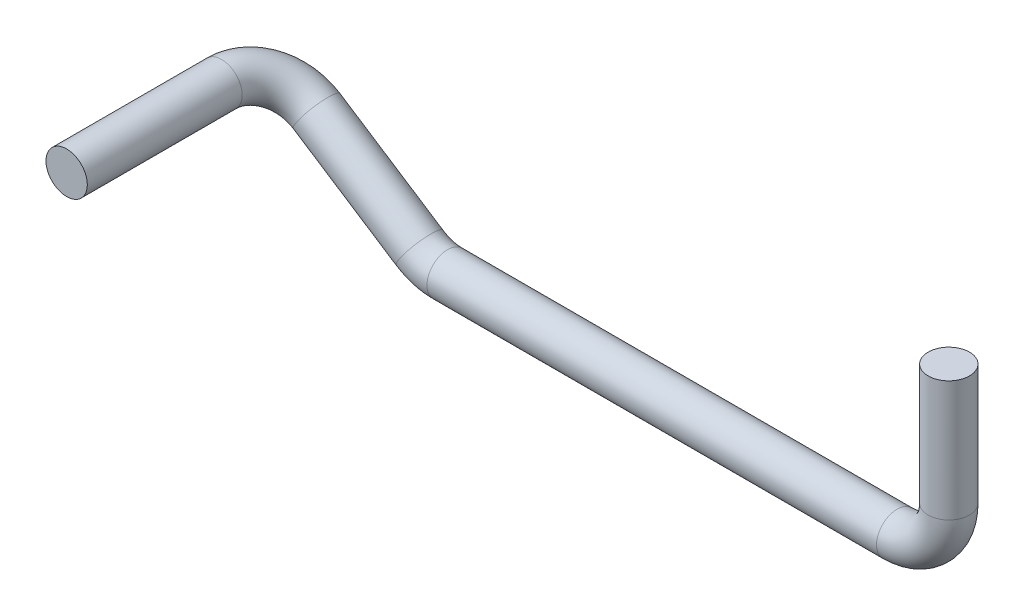
SolidWorks part; units mm, degrees
ref_plane "前视基准面" through (0, 0, 0) normal (0, 0, 1) x (1, 0, 0)
ref_plane "上视基准面" through (0, 0, 0) normal (0, 1, 0) x (1, 0, 0)
ref_plane "右视基准面" through (0, 0, 0) normal (1, 0, 0) x (0, 0, -1)
sketch3d "3D草图1"
  line L0 (4.4429, 0, 0) -> (135, 0, 0)
  line L1 (150, 15, 0) -> (150, 50, 0)
  line L2 (-3.7262, 2.4197, 0) -> (-33.6189, 21.8308, 0)
  line L3 (-46.1992, 30, 15) -> (-46.1992, 30, 60)
  arc A0 (-33.6189, 21.8308, 0) -> (-46.1992, 30, 15) centre (-33.6189, 21.8308, 15) ccw
  arc A1 (4.4429, 0, 0) -> (-3.7262, 2.4197, 0) centre (4.4429, 15, 0) ccw
  arc A2 (135, 0, 0) -> (150, 15, 0) centre (135, 15, 0) ccw
  point P8 (-46.1992, 30, 0)
  point P9 (-25.4497, 34.4111, 15)
  point P12 (0, 0, 0)
  point P13 (4.4429, 15, -15)
  point P16 (150, 0, 0)
  point P17 (135, 15, 15)
  dimension "D5" = 15
  dimension "D6" = 15
  dimension "D7" = 15
  dimension "D1" = 150
  dimension "D2" = 50
  dimension "D3" = 60
  dimension "D4" = 30
sweep "扫描1" add path "3D草图1" circular profile diameter 12 parameters "D3"=12
